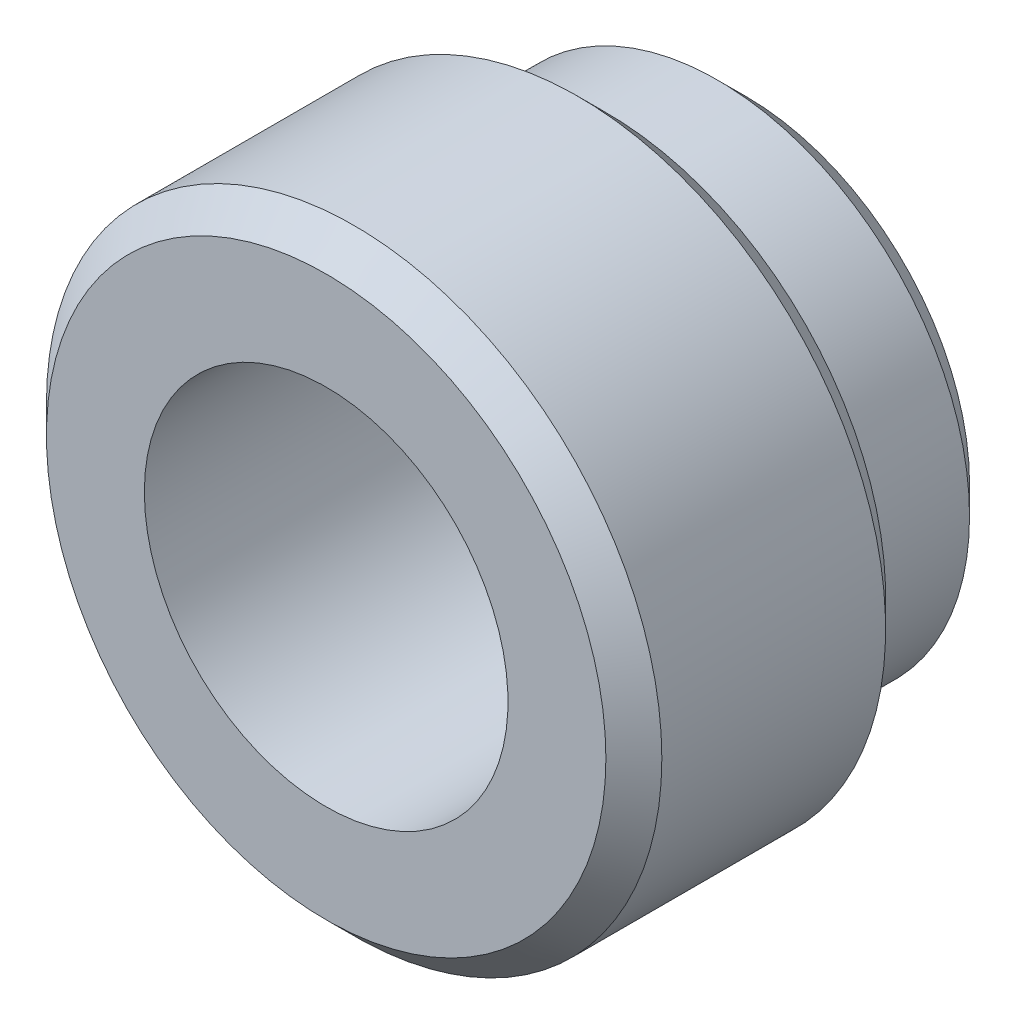
SolidWorks part; units mm, degrees
ref_plane "Front Plane" through (0, 0, 0) normal (0, 0, 1) x (1, 0, 0)
ref_plane "Top Plane" through (0, 0, 0) normal (0, 1, 0) x (1, 0, 0)
ref_plane "Right Plane" through (0, 0, 0) normal (1, 0, 0) x (0, 0, -1)
sketch "Sketch1" plane through (0, 0, 0) normal (0, 0, 1) x (1, 0, 0)
  circle A0 centre (0, 0) radius 11
  dimension "D1" = 22
extrude "Boss-Extrude1" add sketch "Sketch1" along normal blind 15
sketch "Sketch2" plane through (0, 0, 0) normal (0, 0, -1) x (-1, 0, 0)
  circle A0 centre (0, 0) radius 9
  circle A1 centre (0, 0) radius 11
  dimension "D1" = 18
extrude "Cut-Extrude1" cut sketch "Sketch2" against normal blind 5
sketch "Sketch3" plane through (0, 0, 0) normal (0, 0, -1) x (-1, 0, 0)
  circle A0 centre (0, 0) radius 6.5
extrude "Cut-Extrude2" cut sketch "Sketch3" against normal through all
chamfer "Chamfer1" distance 1 angle 45 3 edges at (11, 0, 15) (-11, 0, 5) (-9, 0, 0)
